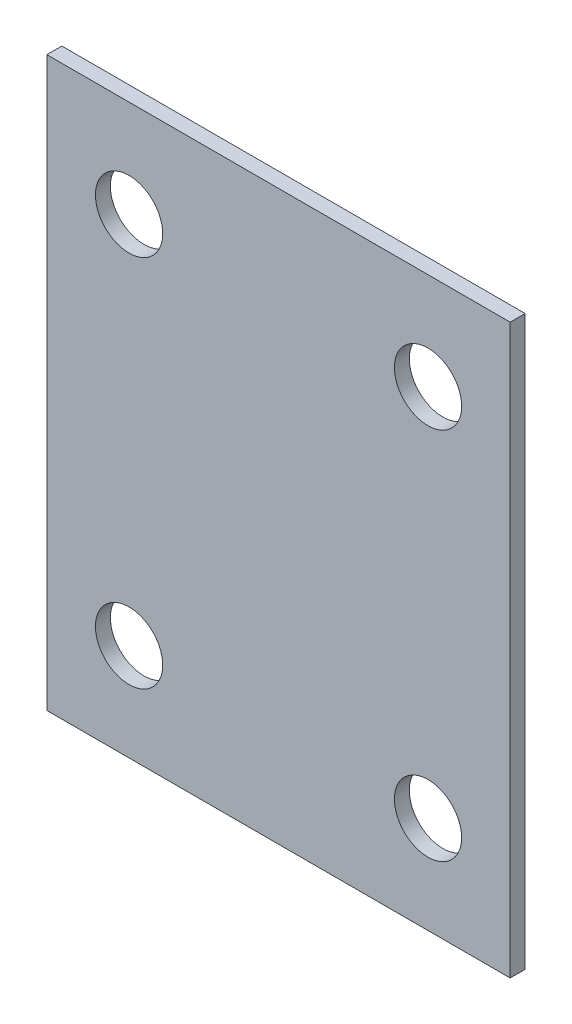
from build123d import *

# Parameters (mm, degrees)
SKETCH_1_W      = 31
SKETCH_1_H      = 38
SKETCH_1_R      = 2.25
EXTRUDE_1_DEPTH = 1


with BuildPart() as part:
    # 草图1 → 凸台-拉伸1 (new body)
    with BuildSketch(Plane.XY):
        Rectangle(SKETCH_1_W, SKETCH_1_H)
        with Locations((-10, 12.5)):
            Circle(SKETCH_1_R, mode=Mode.SUBTRACT)
        with Locations((10, 12.5)):
            Circle(SKETCH_1_R, mode=Mode.SUBTRACT)
        with Locations((10, -12.5)):
            Circle(SKETCH_1_R, mode=Mode.SUBTRACT)
        with Locations((-10, -12.5)):
            Circle(SKETCH_1_R, mode=Mode.SUBTRACT)
    extrude(amount=EXTRUDE_1_DEPTH)


solid = part.part
